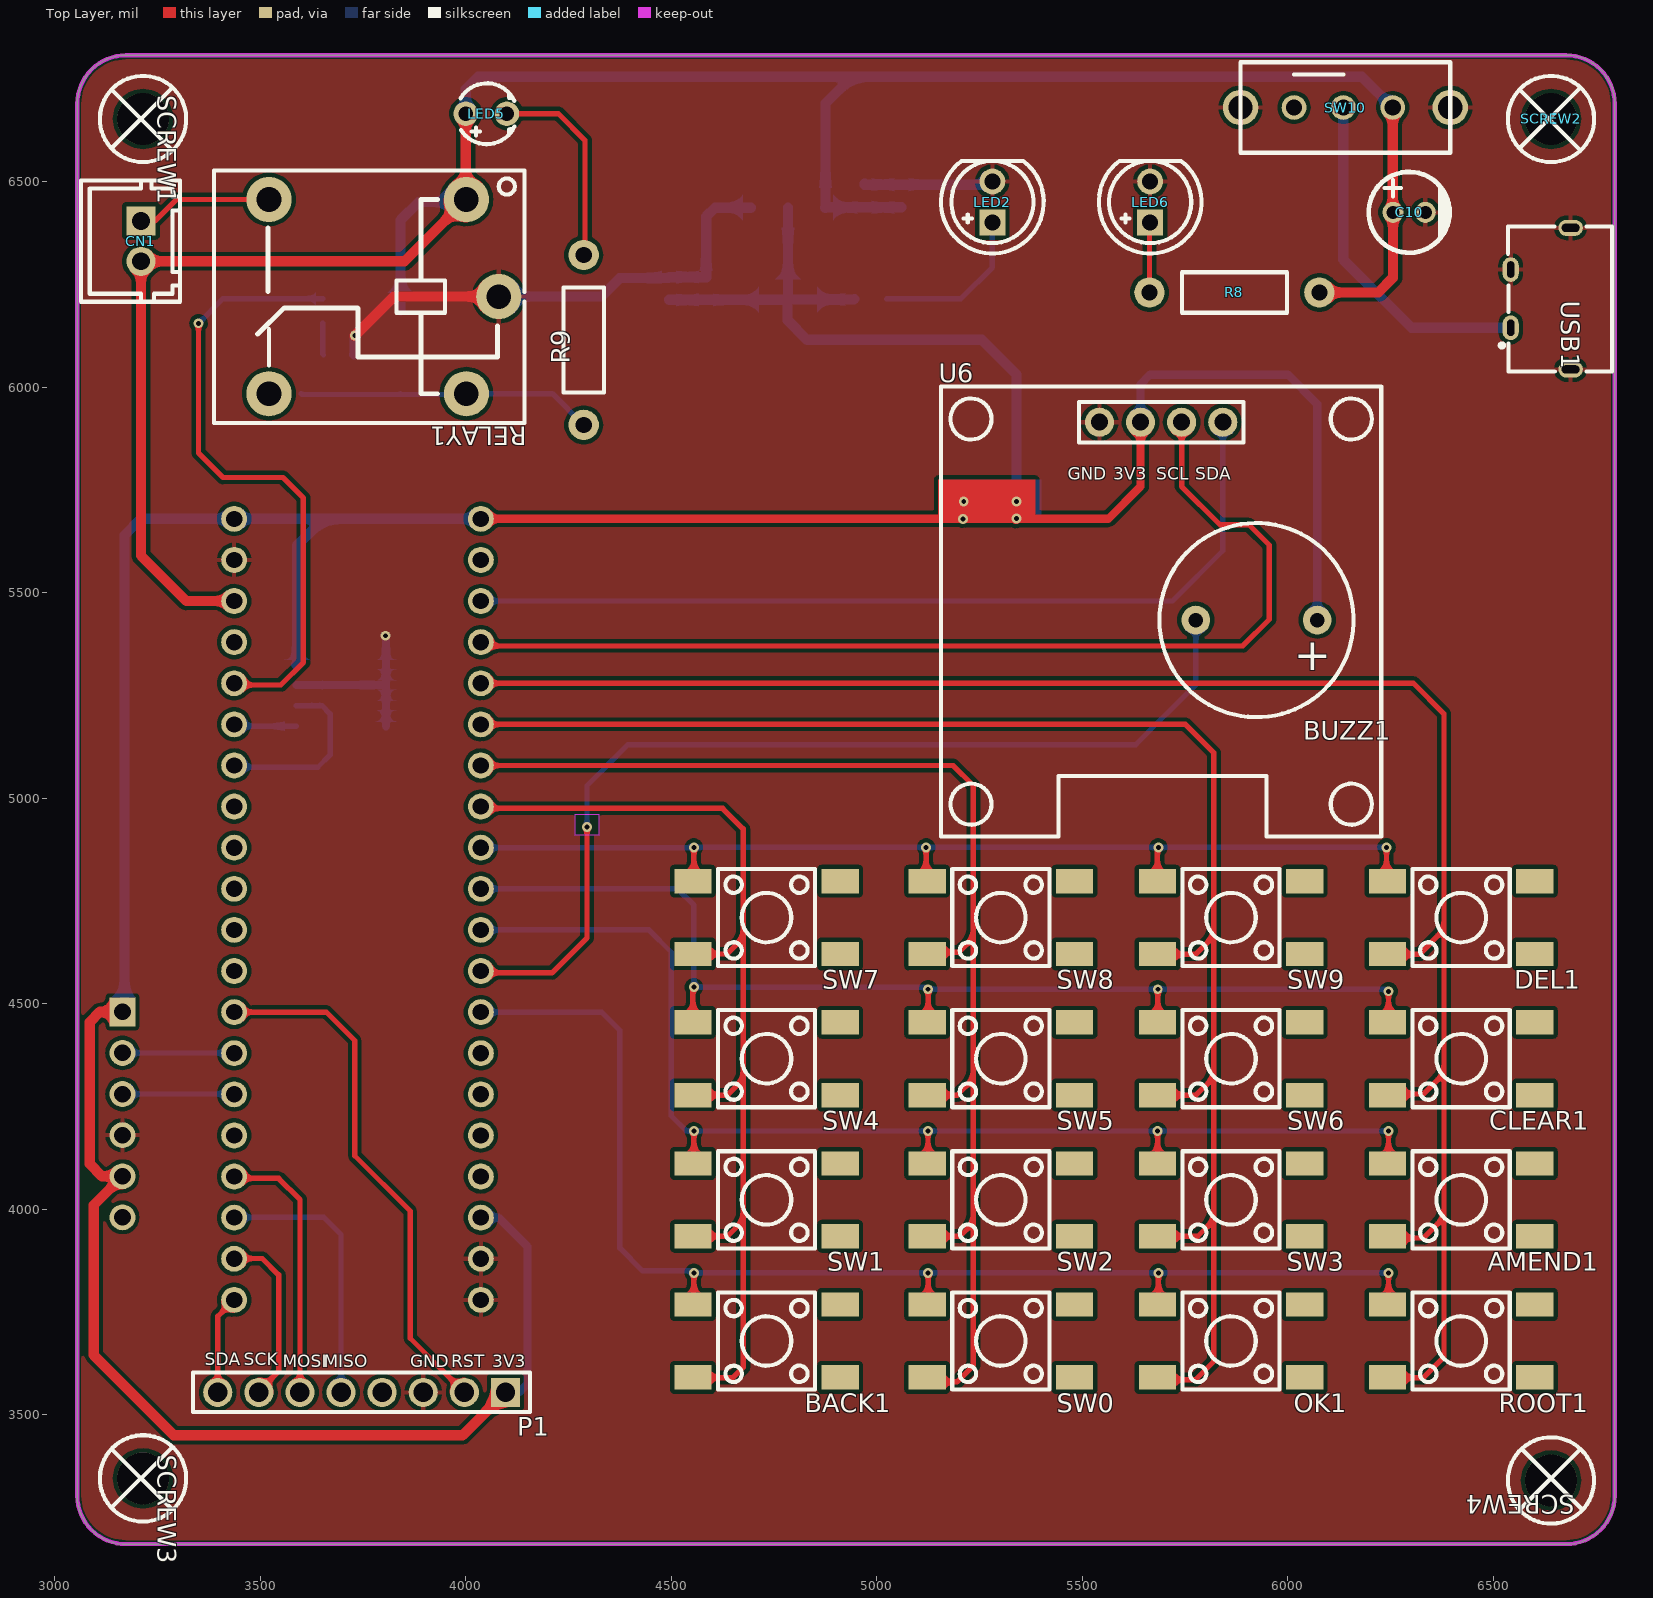
[diagram p0: Top Layer view]
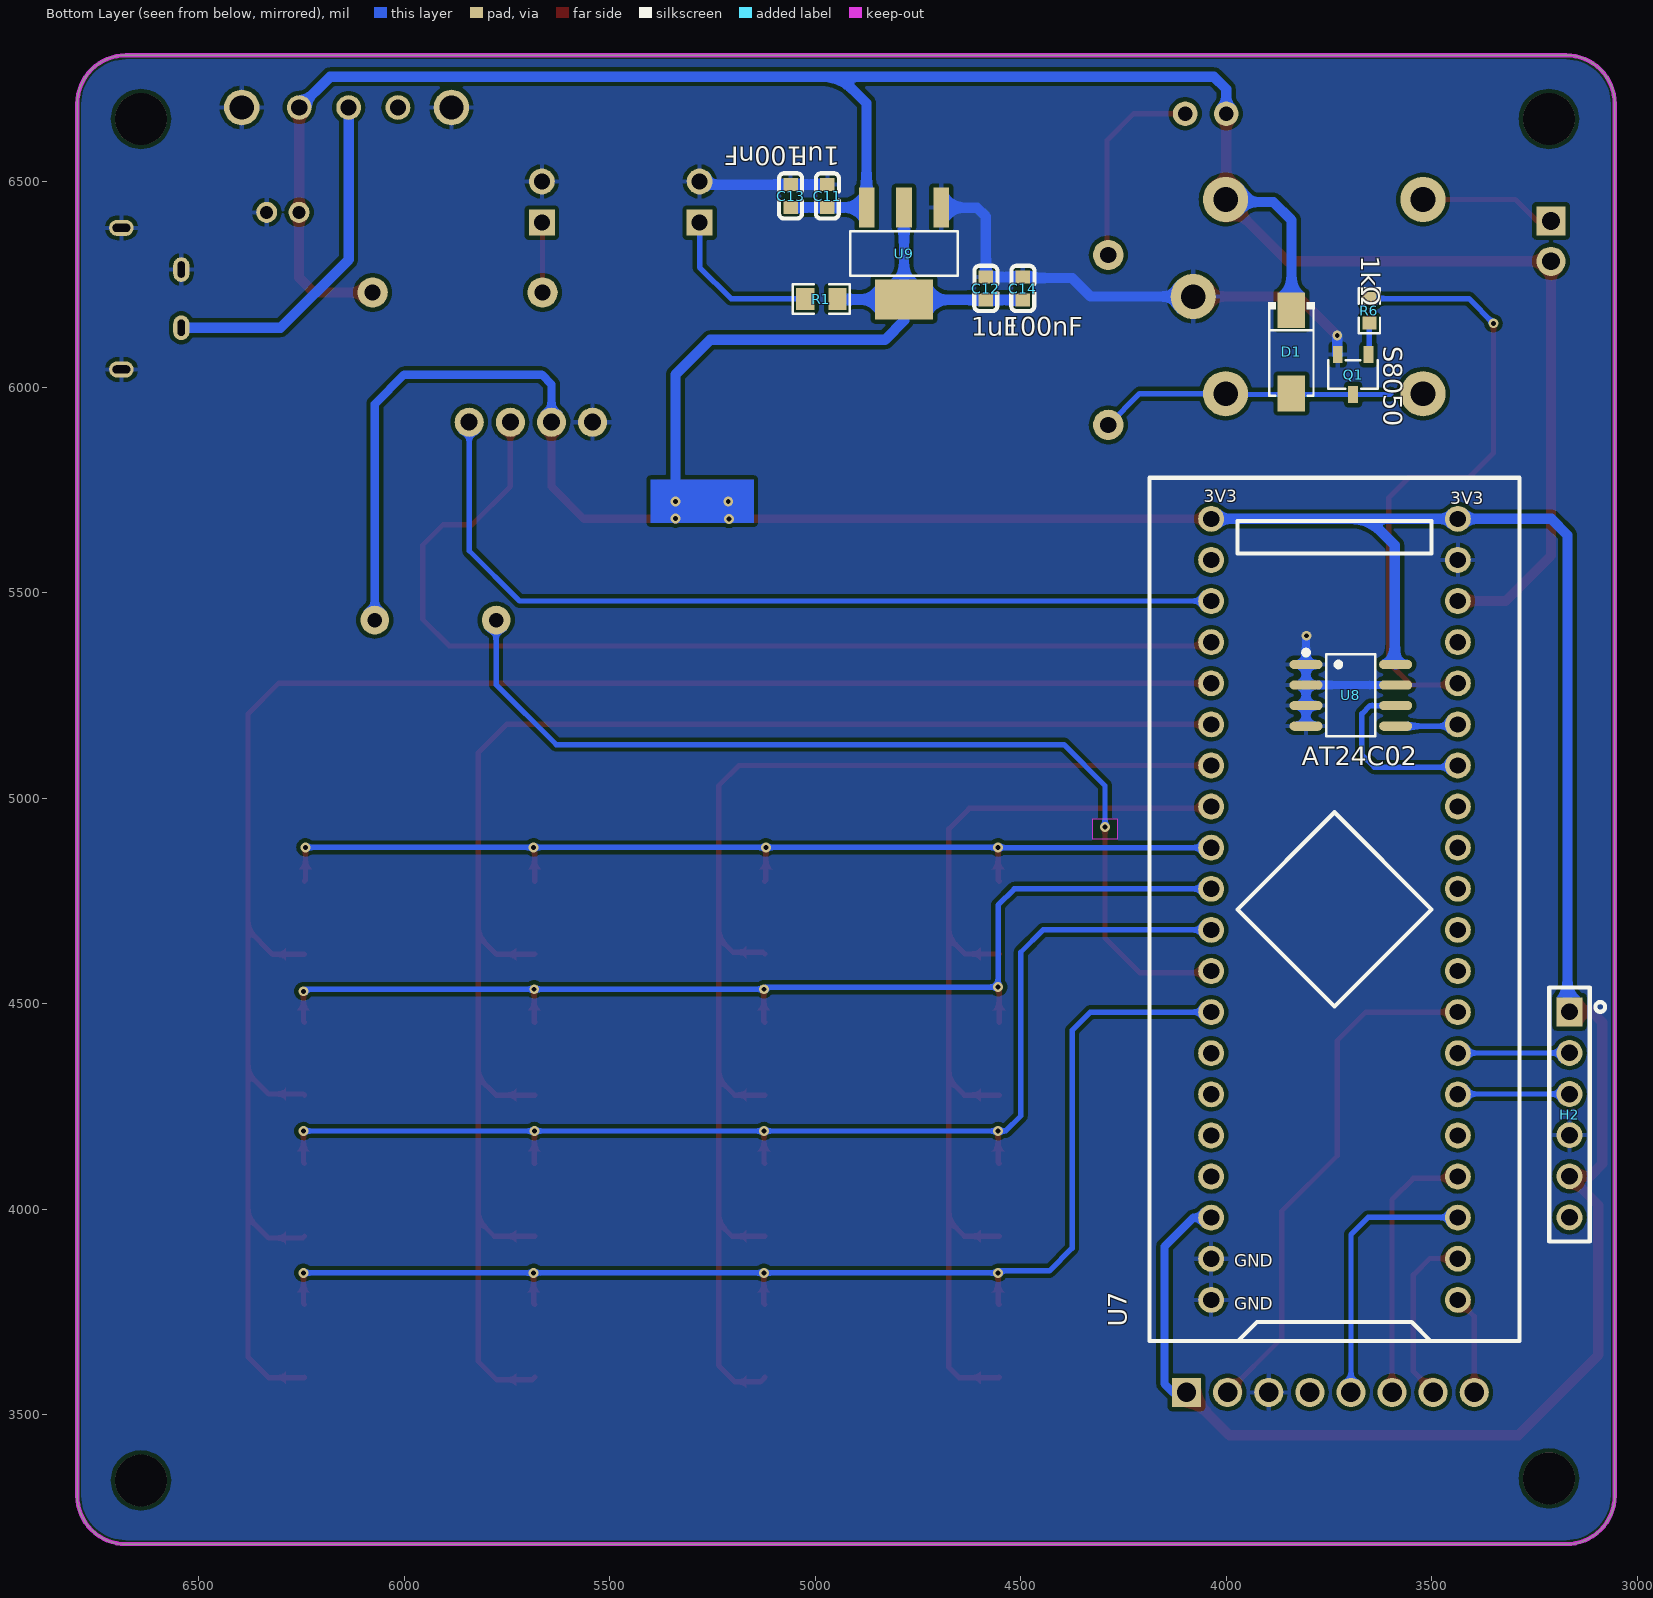
[diagram p1: Bottom Layer view, seen from below]
# Altium PCB MISC61668.pcbdoc
Units mil, origin at the board's own origin, x right, y up, seen from the top; angles counter-clockwise.
Board outline 3740.16 x 3622.05 mil, 2 copper layers (Top Layer, Bottom Layer), stack 62.206 mil thick; 45 components, 31 nets, 185 pads, 24 vias.

## Layer stack, top to bottom
Top Solder Mask Layer: solder mask 0.394, Dk 3.3
Top Layer: signal copper 1.379
Dielectric1: surface 59.449, FR4, Dk 4.5
Bottom Layer: signal copper 1.378
Bottom Solder Mask Layer: solder mask 0.394, Dk 3.3

## Board outline
3173.11,6807.05 ccw(c3173.11,6688.94) 3055,6688.94 3055,3303.11 ccw(c3173.11,3303.11) 3173.11,3185 6677.05,3185 ccw(c6677.05,3303.11) 6795.16,3303.11 6795.16,6688.94 ccw(c6677.05,6688.94) 6677.05,6807.05

## Design rules (kind name [scope] priority, off if disabled: settings)
BoardOutlineClearance copperThickness2oz_1 [All] p2 off: genericclearance=8 ignorepadtopadclearanceinfootprint=FALSE except(0: Arc-SplitContinuation Track-SplitContinuation SMDPad-SplitContinuation THPad-SplitContinuation Via-SplitContinuation Fill-SplitContinuation Region-SplitContinuation Poly-SplitContinuation Text-SplitContinuation Hole-SplitContinuation; 6: Arc-OutlineEdge Track-OutlineEdge SMDPad-OutlineEdge THPad-OutlineEdge Via-OutlineEdge Fill-OutlineEdge Region-OutlineEdge Text-OutlineEdge Hole-OutlineEdge Arc-CutoutEdge Track-CutoutEdge SMDPad-CutoutEdge THPad-CutoutEdge Via-CutoutEdge Fill-CutoutEdge Region-CutoutEdge Text-CutoutEdge Hole-CutoutEdge; 10: Poly-OutlineEdge Poly-CutoutEdge)
BoardOutlineClearance Plane_innerPlane_1 [All] p4 off: genericclearance=8 ignorepadtopadclearanceinfootprint=FALSE except(0: Arc-SplitContinuation Track-SplitContinuation SMDPad-SplitContinuation THPad-SplitContinuation Via-SplitContinuation Fill-SplitContinuation Region-SplitContinuation Poly-SplitContinuation Text-SplitContinuation Hole-SplitContinuation; 6: Arc-OutlineEdge SMDPad-OutlineEdge THPad-OutlineEdge Via-OutlineEdge Fill-OutlineEdge Region-OutlineEdge Text-OutlineEdge Hole-OutlineEdge Arc-CutoutEdge SMDPad-CutoutEdge THPad-CutoutEdge Via-CutoutEdge Fill-CutoutEdge Region-CutoutEdge Text-CutoutEdge Hole-CutoutEdge; 8: Track-OutlineEdge Track-CutoutEdge; 10: Poly-OutlineEdge Poly-CutoutEdge)
BoardOutlineClearance Copper_copperRegion_1 [All] p6 off: genericclearance=8 ignorepadtopadclearanceinfootprint=FALSE except(0: Arc-SplitContinuation Track-SplitContinuation SMDPad-SplitContinuation THPad-SplitContinuation Via-SplitContinuation Fill-SplitContinuation Region-SplitContinuation Poly-SplitContinuation Text-SplitContinuation Hole-SplitContinuation; 6: Arc-OutlineEdge SMDPad-OutlineEdge THPad-OutlineEdge Via-OutlineEdge Fill-OutlineEdge Region-OutlineEdge Text-OutlineEdge Hole-OutlineEdge Arc-CutoutEdge SMDPad-CutoutEdge THPad-CutoutEdge Via-CutoutEdge Fill-CutoutEdge Region-CutoutEdge Text-CutoutEdge Hole-CutoutEdge; 8: Track-OutlineEdge Track-CutoutEdge; 10: Poly-OutlineEdge Poly-CutoutEdge)
BoardOutlineClearance copperThickness1oz_1 [All] p8: genericclearance=8 ignorepadtopadclearanceinfootprint=FALSE except(0: Arc-SplitContinuation Track-SplitContinuation SMDPad-SplitContinuation THPad-SplitContinuation Via-SplitContinuation Fill-SplitContinuation Region-SplitContinuation Poly-SplitContinuation Text-SplitContinuation Hole-SplitContinuation; 6: Arc-OutlineEdge SMDPad-OutlineEdge THPad-OutlineEdge Via-OutlineEdge Fill-OutlineEdge Region-OutlineEdge Text-OutlineEdge Hole-OutlineEdge Arc-CutoutEdge SMDPad-CutoutEdge THPad-CutoutEdge Via-CutoutEdge Fill-CutoutEdge Region-CutoutEdge Text-CutoutEdge Hole-CutoutEdge; 8: Track-OutlineEdge Track-CutoutEdge; 10: Poly-OutlineEdge Poly-CutoutEdge)
Clearance copperThickness2oz [All] p1 off: gap=8 ignorepadtopadclearanceinfootprint=FALSE except(6: SMDPad-Track SMDPad-SMDPad THPad-Track SMDPad-THPad THPad-THPad Track-Via SMDPad-Via THPad-Via Via-Via Fill-Track Region-Track Fill-SMDPad Region-SMDPad Fill-THPad Region-THPad Fill-Via Region-Via Fill-Fill Fill-Region Region-Region Arc-SMDPad Arc-THPad Arc-Via Fill-Arc Region-Arc Arc-Arc Text-Track SMDPad-Text Text-THPad Text-Via Fill-Text Region-Text Text-Text Hole-Track Hole-SMDPad Hole-THPad Hole-Via Fill-Hole Region-Hole Hole-Arc Hole-Text; 10: Poly-Track Poly-SMDPad Poly-THPad Poly-Via Poly-Fill Poly-Region Poly-Poly Poly-Arc Poly-Text Poly-Hole; 11.8: Arc-Track Arc-Text)
Clearance Plane_innerPlane [All] p3 off: gap=8 ignorepadtopadclearanceinfootprint=FALSE except(6: SMDPad-SMDPad SMDPad-THPad THPad-THPad SMDPad-Via THPad-Via Via-Via Fill-SMDPad Region-SMDPad Fill-THPad Region-THPad Fill-Via Region-Via Fill-Fill Fill-Region Region-Region Arc-SMDPad Arc-THPad Arc-Via Fill-Arc Region-Arc Arc-Arc SMDPad-Text Text-THPad Text-Via Fill-Text Region-Text Text-Text Hole-SMDPad Hole-THPad Hole-Via Fill-Hole Region-Hole Hole-Arc Hole-Text; 10: Poly-Track Poly-SMDPad Poly-THPad Poly-Via Poly-Fill Poly-Region Poly-Poly Poly-Arc Poly-Text Poly-Hole; 11.8: Arc-Text)
Clearance Copper_copperRegion [All] p5 off: gap=8 ignorepadtopadclearanceinfootprint=FALSE except(6: SMDPad-SMDPad SMDPad-THPad THPad-THPad SMDPad-Via THPad-Via Via-Via Fill-SMDPad Region-SMDPad Fill-THPad Region-THPad Fill-Via Region-Via Fill-Fill Fill-Region Region-Region Arc-SMDPad Arc-THPad Arc-Via Fill-Arc Region-Arc Arc-Arc SMDPad-Text Text-THPad Text-Via Fill-Text Region-Text Text-Text Hole-SMDPad Hole-THPad Hole-Via Fill-Hole Region-Hole Hole-Arc Hole-Text; 10: Poly-Track Poly-SMDPad Poly-THPad Poly-Via Poly-Fill Poly-Region Poly-Poly Poly-Arc Poly-Text Poly-Hole; 11.8: Arc-Text)
Clearance copperThickness1oz [All] p7: gap=8 ignorepadtopadclearanceinfootprint=FALSE except(6: SMDPad-SMDPad SMDPad-THPad THPad-THPad SMDPad-Via THPad-Via Via-Via Fill-SMDPad Region-SMDPad Fill-THPad Region-THPad Fill-Via Region-Via Fill-Fill Fill-Region Region-Region Arc-SMDPad Arc-THPad Arc-Via Fill-Arc Region-Arc Arc-Arc SMDPad-Text Text-THPad Text-Via Fill-Text Region-Text Text-Text Hole-SMDPad Hole-THPad Hole-Via Fill-Hole Region-Hole Hole-Arc Hole-Text; 10: Poly-Track Poly-SMDPad Poly-THPad Poly-Via Poly-Fill Poly-Region Poly-Poly Poly-Arc Poly-Text Poly-Hole; 11.8: Arc-Text)
DiffPairsRouting differentialPair [All] p1: maxlimit=6 minlimit=6 mostfreqgap=6 toplayer_minwidth=5 toplayer_prefwidth=10 toplayer_maxwidth=100 toplayer_mingap=6 toplayer_prefgap=6 toplayer_maxgap=6 bottomlayer_minwidth=5 bottomlayer_prefwidth=10 bottomlayer_maxwidth=100 bottomlayer_mingap=6 bottomlayer_prefgap=6 bottomlayer_maxgap=6 maxuncoupledlength=10
HoleToHoleClearance otherClearance [All] p1: gap=11.8 allowstackedmicrovias=TRUE
Length netLength [All] p1: minlimit=0 maxlimit=0
PasteMaskExpansion pasteMaskExpansion [All] p1: expansion=0
PlaneConnect innerPlane [All] p1: planeconnectstyle=Relief reliefexpansion=20 reliefentries=4 reliefconductorwidth=10 reliefairgap=10
PolygonConnect copperRegion [All] p1: connectstyle=Relief reliefconductorwidth=10 reliefentries=4 polygonreliefangle="90 Angle" airgapwidth=10 via.connectstyle=Relief via.reliefconductorwidth=10 via.reliefentries=4 via.polygonreliefangle="90 Angle" via.airgapwidth=10
RoutingVias viaSize [All] p1: holewidth=12 width=24 viastyle="Through Hole" minholewidth=11.8 minwidth=19.7 maxholewidth=248 maxwidth=393.7
SolderMaskExpansion solderMaskExpansion [IsVia] p1: expansion=-1000 istentingtop=TRUE
SolderMaskExpansion solderMaskExpansion [All] p2: expansion=2 istentingtop=FALSE
Width copperThickness2oz_2 [(InNet('+3V3') OR InNet('+5V') OR InNet('GND'))] p1: maxlimit=100 minlimit=8 preferedwidth=25
Width copperThickness1oz_2 [All] p2: maxlimit=100 minlimit=5 preferedwidth=13

## Components (designator, comment, footprint, x,y, rotation, side; value= is the part's Value field where it differs from the comment)
AMEND1 "KH-6X6X5H-STM" SW-SMD_4P-L6.0-W6.0-P4.50-LS9.0-2 6421.7,4022.66 r180 top
BACK1 "KH-6X6X5H-STM" SW-SMD_4P-L6.0-W6.0-P4.50-LS9.0-2 4731.7,3679.33 r180 top
BUZZ1 "Buzzer BD12.0-P7.50" BUZ-TH_BD12.0-P7.50-D0.6-FD 5923.78,5433.05 r180 top
C10 "10uF" CAP-TH_BD5.0-P2.00-D0.8-FD 6295,6425 r0 top
C11 "1uF" C0603 4970.55,6464.66 r270 bottom
C12 "1uF" C0603 4585,6239.66 r270 bottom
C13 "100nF" C0603 5060,6464.66 r270 bottom
C14 "100nF" C0603 4495,6239.66 r270 bottom
CLEAR1 "KH-6X6X5H-STM" SW-SMD_4P-L6.0-W6.0-P4.50-LS9.0-2 6421.7,4365.99 r180 top
CN1 "ZX-XH2.54-2PZZ" CONN-TH_2P-P2.50_HX25003-2A 3210,6355 r270 top
D1 "SS14" SMA_L4.2-W2.6-LS5.3-RD 3841.48,6085.3 r270 bottom
DEL1 "KH-6X6X5H-STM" SW-SMD_4P-L6.0-W6.0-P4.50-LS9.0-2 6421.7,4709.33 r180 top
H2 "PM254V-11-06-H85" hdr-th_6p-p2.54-v-f 3165,4230 r270 bottom
LED2 "" LED-TH_5mm 5281.16,6450 r90 top
LED5 "XL-302SURD" LED-TH_BD3.8-P2.54-RD 4050,6665 r180 top
LED6 "" LED-TH_5mm 5665,6450 r90 top
OK1 "KH-6X6X5H-STM" SW-SMD_4P-L6.0-W6.0-P4.50-LS9.0-2 5861.7,3679.33 r180 top
P1 "2.54-1*8P female, RoHS" HDR-TH_8P-P2.54-V-F-1 3746.7,3554.33 r180 top
Q1 "S8050" SOT-23-3_L2.9-W1.6-P1.90-LS2.8-BR 3691.48,6030.3 r90 bottom
R1 "10.1kΩ" R0805 4985,6214.05 r0 bottom
R6 "1kΩ" R0603 3652.01,6185.3 r90 bottom
R8 "1kΩ" RES-TH_BD2.5-L6.5-P10.50-D0.6 5870,6230 r180 top
R9 "1kΩ" RES-TH_BD2.5-L6.5-P10.50-D0.6 4286.91,6114.55 r90 top
RELAY1 "SRD-12VDC-SL-C" RELAY-TH_SRD-XXVDC-XL-C 3800.77,6220.03 r180 top locked
ROOT1 "KH-6X6X5H-STM" SW-SMD_4P-L6.0-W6.0-P4.50-LS9.0-2 6421.7,3679.33 r180 top
SCREW1 "" M3螺丝 3212.48,6649.57 r270 top locked
SCREW2 "" M3螺丝 6637.68,6649.57 r270 top locked
SCREW3 "" M3螺丝 3212.48,3342.48 r270 top locked
SCREW4 "" M3螺丝 6637.68,3342.48 r180 top locked
SW0 "KH-6X6X5H-STM" SW-SMD_4P-L6.0-W6.0-P4.50-LS9.0-2 5301.7,3679.33 r180 top
SW1 "KH-6X6X5H-STM" SW-SMD_4P-L6.0-W6.0-P4.50-LS9.0-2 4731.7,4022.66 r180 top
SW2 "KH-6X6X5H-STM" SW-SMD_4P-L6.0-W6.0-P4.50-LS9.0-2 5301.7,4022.66 r180 top
SW3 "KH-6X6X5H-STM" SW-SMD_4P-L6.0-W6.0-P4.50-LS9.0-2 5861.7,4022.66 r180 top
SW4 "KH-6X6X5H-STM" SW-SMD_4P-L6.0-W6.0-P4.50-LS9.0-2 4731.7,4365.99 r180 top
SW5 "KH-6X6X5H-STM" SW-SMD_4P-L6.0-W6.0-P4.50-LS9.0-2 5301.7,4365.99 r180 top
SW6 "KH-6X6X5H-STM" SW-SMD_4P-L6.0-W6.0-P4.50-LS9.0-2 5861.7,4365.99 r180 top
SW7 "KH-6X6X5H-STM" SW-SMD_4P-L6.0-W6.0-P4.50-LS9.0-2 4731.7,4709.33 r180 top locked
SW8 "KH-6X6X5H-STM" SW-SMD_4P-L6.0-W6.0-P4.50-LS9.0-2 5301.7,4709.33 r180 top
SW9 "KH-6X6X5H-STM" SW-SMD_4P-L6.0-W6.0-P4.50-LS9.0-2 5861.7,4709.33 r180 top
SW10 "SK-12E12-G5" SW-TH_SK-12E12-G5 6140,6680 r90 top
U6 "HS96L03W2C03" OLED-TH_L27.8-W27.2-P2.54_C9900033791 5691.7,5914.33 r0 top
U7 "STM32F103C8T6-Card" CONN-TH_L53.3-W22.9_STM32F103C8T6-CARD 3736.7,4729.33 r90 bottom locked
U8 "AT24C02" SOP-8_L5.0-W4.0-P1.27-LS6.0-BL 3696.96,5250 r270 bottom
U9 "AMS1117-3.3" SOT-223-4_L6.5-W3.5-P2.30-LS7.0-BR 4783.95,6324.77 r90 bottom
USB1 "KH-TYPE-C-2P" USB-SMD_KH-TYPE-C-2P 6615,6215 r90 top

## Footprints (in the part's own frame and the unit in brackets; to place one, negate y for a bottom-side part, rotate by r counter-clockwise, add the part's x,y. Pads: shape width x height; smd on the part's side, far side on the other; paste and mask are expansions set on the pad)
BUZ-TH_BD12.0-P7.50-D0.6-FD [mil]
  round 70 hole 35.43: 1(-147.64,0) 2(147.64,0)
  silkscreen extent -236,-236 236,236
C0603 [mm]
  rect 0.8x0.9 smd: 1(-0.7,0) 2(0.7,0)
  silkscreen extent -1.41,-0.71 1.39,0.72
CAP-TH_BD5.0-P2.00-D0.8-FD [mm]
  round 1.3 hole 0.8: 1(-1,0) 2(1,0)
  silkscreen extent -2.5,-2.5 2.5,2.5
CONN-TH_2P-P2.50_HX25003-2A [mm]
  rect 1.8x1.8 hole 1.1 paste+0 mask+0.05: 1(-1.25,0)
  round 1.8 hole 1.1 paste+0 mask+0.05: 2(1.25,0)
  silkscreen extent -3.75,-3.7 3.75,2.41
CONN-TH_L53.3-W22.9_STM32F103C8T6-CARD [mm]
  round 1.6 hole 1: 1(-24.13,-7.62) 2(-21.59,-7.62) 3(-19.05,-7.62) 4(-16.51,-7.62) 5(-13.97,-7.62) 6(-11.43,-7.62) 7(-8.89,-7.62) 8(-6.35,-7.62) 9(-3.81,-7.62) 10(-1.27,-7.62) 11(1.27,-7.62) 12(3.81,-7.62) 13(6.35,-7.62) 14(8.89,-7.62) 15(11.43,-7.62) 16(13.97,-7.62) 17(16.51,-7.62) 18(19.05,-7.62) 19(21.59,-7.62) 20(24.13,-7.62) 21(24.13,7.62) 22(21.59,7.62) 23(19.05,7.62) 24(16.51,7.62) 25(13.97,7.62) 26(11.43,7.62) 27(8.89,7.62) 28(6.35,7.62) 29(3.81,7.62) 30(1.27,7.62) 31(-1.27,7.62) 32(-3.81,7.62) 33(-6.35,7.62) 34(-8.89,7.62) 35(-11.43,7.62) 36(-13.97,7.62) 37(-16.51,7.62) 38(-19.05,7.62) 39(-21.59,7.62) 40(-24.13,7.62)
  silkscreen extent -26.67,-11.43 26.67,11.43
hdr-th_6p-p2.54-v-f [mm]
  rect 1.8x1.6 hole 1.02: 1(-6.35,0)
  round 1.6 hole 1.02: 2(-3.81,0) 3(-1.27,0) 4(1.27,0) 5(3.81,0) 6(6.35,0)
  silkscreen extent -7.85,-1.25 7.85,2.2
HDR-TH_8P-P2.54-V-F-1 [mm]
  rect 1.8x1.8 hole 1.2: 1(-8.89,0)
  round 1.8 hole 1.2: 2(-6.35,0) 3(-3.81,0) 4(-1.27,0) 5(1.27,0) 6(3.81,0) 7(6.35,0) 8(8.89,0)
  silkscreen extent -10.41,-1.22 10.41,1.22
LED-TH_5mm [mm]
  rect 1.6x1.6 hole 1 paste+0 mask+0.051: 1(-1.27,0)
  round 1.6 hole 1 paste+0 mask+0.051: 2(1.27,0)
  silkscreen extent -3.17,-3.17 2.54,3.17
LED-TH_BD3.8-P2.54-RD [mil]
  round 60 hole 35.43: 1(-50,0) 2(50,0)
  silkscreen extent -68,-74 63,74
M3螺丝 [mil]
  round 126 hole 126 paste+0 mask+4: 1(-2.5,2.5)
  silkscreen extent -107,-102 102,107
OLED-TH_L27.8-W27.2-P2.54_C9900033791 [mm]
  round 1.8 hole 1.05 paste+0 mask+0.05: 1(-3.81,0) 2(-1.27,0) 3(1.27,0) 4(3.81,0)
  silkscreen extent -13.6,-25.6 13.6,2.2
R0603 [mil]
  rect 31.75x34.02 smd paste-3937.01 mask+2: 1(-29.66,0) 2(29.66,0)
  silkscreen extent -55,-26 55,26
R0805 [mm]
  rect 1.133x1.377 smd paste-100 mask+0.051: 1(-1,0) 2(1,0)
  silkscreen extent -1.76,-0.92 1.76,0.92
RELAY-TH_SRD-XXVDC-XL-C [mil]
  round 110 hole 60: 1(-200.79,-236.22) 2(279.53,-236.2) 3(279.53,236.2) 4(-200.79,236.22) 5(-279.53,0)
  silkscreen extent -342,-307 413,307
RES-TH_BD2.5-L6.5-P10.50-D0.6 [mil]
  round 74 hole 39.37: 1(-206.69,0) 2(206.69,0)
  silkscreen extent -128,-49 128,49
SMA_L4.2-W2.6-LS5.3-RD [mm]
  rect 2.2x1.7 smd: 1(-2.565,0) 2(2.565,0)
  silkscreen extent -3.08,-1.44 2.7,1.44
SOP-8_L5.0-W4.0-P1.27-LS6.0-BL [mil]
  oval 22.6x80.14 smd: 1(-75,-108.97) 2(-25,-108.97) 3(25,-108.97) 4(75,-108.97) 5(75,108.97) 6(25,108.97) 7(-25,108.97) 8(-75,108.97)
  silkscreen extent -110,-115 99,60
SOT-23-3_L2.9-W1.6-P1.90-LS2.8-BR [mm]
  rect 1.07x0.6 smd: 1(1.235,-0.95) 2(1.235,0.95) 3(-1.235,0)
  silkscreen extent -0.88,-1.54 0.88,1.54
SOT-223-4_L6.5-W3.5-P2.30-LS7.0-BR [mm]
  rect 2.47x0.98 smd: 1(2.835,-2.3) 2(2.835,0) 3(2.835,2.3)
  rect 2.47x3.6 smd: 4(-2.835,0)
  silkscreen extent -1.37,-3.33 1.37,3.33
SW-SMD_4P-L6.0-W6.0-P4.50-LS9.0-2 [mm]
  rect 2.3x1.5 smd: 1(-4.55,2.25) 2(4.55,2.25) 3(-4.55,-2.25) 4(4.55,-2.25)
  silkscreen extent -3,-3 3,3
SW-TH_SK-12E12-G5 [mil]
  round 60 hole 39.37: 1(0,125) 2(0,5) 3(0,-115)
  round 86.61 hole 59.06: 4(0,-255) 5(0,255)
  silkscreen extent -110,-255 110,255
USB-SMD_KH-TYPE-C-2P [mm]
  oval 1.524x1 hole 0.45 slot 1 at 0 deg paste+0 mask+0.05: 1(-1.8,1.85) 2(1.8,1.85)
  oval 1x1.524 hole 0.5 slot 1.1 at 90 deg paste+0 mask+0.05: 3(4.375,-1.85) 4(-4.375,-1.85)
  silkscreen extent -4.5,-4.41 4.46,2.53

## Via types
v1: diameter 24, hole 12, Top Layer to Bottom Layer, 24 vias

## Nets (pads, with @x,y where several pads share a name; then routed paths per layer and width w, separated by ;. In a path a pad name is that pad's centre, name@x,y a point inside that pad or via, vN(x,y) a via of type N, cw(c..) or ccw(c..) an arc to the next point about the centre after c; other vN are vias at no path point)
$1N2265: LED2.1 R1.2 | length 397.6
  Bottom Layer w13: R1.2 5025.32,6215 5205,6215 5281.16,6291.16 LED2.1
$1N4836: CN1.1 RELAY1.2 | length 332.8
  Top Layer w13: CN1.1 3244.21,6404.21 3296.23,6456.23 RELAY1.2
$1N5221: D1.2 Q1.3 R9.1 RELAY1.4 | length 723.9
  Bottom Layer w13: 3599.98,5983.81 3602.1,5981.68 Q1.3 D1.2@3838.86,5981.68 ; D1.2 D1.2@3838.86,5981.68 ; R9.1 4210.96,5983.81 RELAY1.4 3999.43,5981.68 D1.2@3838.86,5981.68
$1N5245: Q1.1 R6.1 | length 77.6
  Bottom Layer w13: R6.1 3652.01,6081 Q1.1
$1N11459: SW10.2 USB1.1 | length 845.9
  Bottom Layer w25: SW10.2 6135,6310 6300.87,6144.13 USB1.1
$1N11461: LED6.1 R8.2 | length 170.7
  Top Layer w13: R8.2 5663.31,6398.31 LED6.1
$1N12136: LED5.1 R9.2 | length 497
  Top Layer w13: LED5.1 4225,6665 4290,6600 4290,6324.33 R9.2
+3V3: BUZZ1.1 C12.2 C14.2 H2.1 H2.5 P1.1 R1.1 U6.2 U7.20 U7.21 U7.38 U8.8 U9.2 U9.4 | length 9651
  Top Layer w20: U7.21 v1(5209.89,5679.33) v1@5337.73,5679.33 ; v1@5339.33,5679.33 5563.05,5679.33 5641.7,5757.97 U6.2
  Top Layer w25: H2.1 3110,4480 3085,4455 3085,4110 3115,4080 H2.5 3095,4010 3095,3645 3290,3450 3992.37,3450 P1.1 ; v1@5337.73,5679.33 5339.33,5679.33 v1(5340,5680)
  Bottom Layer w20: U7.38 4080,3979.33 4150,3909.33 4150,3575 4129.33,3554.33 P1.1 ; U6.2 5641.7,6006.7 5665,6030 6000,6030 6071.42,5958.58 BUZZ1.1
  Bottom Layer w25: H2.1 3170,4485 3170,5640 3209.33,5679.33 U7.20 3654.2,5679.33 ; U8.8 3590,5327.01 3590,5615.13 3654.2,5679.33 ; U7.21 3654.2,5679.33 ; C14.2 C12.2 U9.4@4782.9,6212.1 ; U9.2 U9.4 ; R1.1 4944.74,6213.16 U9.4 ; v1(5340,5680) v1(5340,5721.21) 5340,6030 5255,6115 4830,6115 4782.9,6162.1 U9.4@4782.9,6212.1 ; U9.4@4782.9,6212.1 U9.4
  other v1: 5211.47,5721.21
+5V: C10.1 C11.2 C13.2 CN1.2 D1.1 LED5.2 R8.1 RELAY1.1 SW10.3 U7.18 U9.3 | length 5949.8
  Top Layer w25: U7.18 3320.67,5479.33 3210,5590 CN1.2 3851.1,6305.79 RELAY1.1 4000,6457.8 LED5.2 ; R8.1 6220,6230 6255.63,6265.63 C10.1 6255,6425.63 SW10.3
  Bottom Layer w25: D1.1 3841.48,6406.48 3885,6450 3995.31,6450 RELAY1.1 ; LED5.2 4000,6725 4030,6755 4940,6755 ; U9.3 U9.3@4875.23,6437.1 ; C13.2 C11.2 U9.3@4875.23,6437.1 ; SW10.3 6180,6755 4940,6755 ; U9.3@4875.23,6437.1 4875.23,6690.23 4940,6755
BUZZER_PA7: BUZZ1.2 U7.32 | length 2405.3
  Top Layer w13: U7.32 4041.03,4575 4210,4575 4295,4660 v1(4295,4930)
  Bottom Layer w13: v1(4295,4930) 4295,5030 4395,5130 5630,5130 5776.14,5276.14 BUZZ1.2
GND: C10.2 C11.1 C12.1 C13.1 C14.1 H2.4 LED2.2 LED6.2 P1.3 Q1.2 RELAY1.5 SW10.4 SW10.5 U6.1 U7.19 U7.39 U7.40 U8.1 U8.2 U8.3 U8.4 U8.7 U9.1 USB1.2 USB1.3 USB1.4 | length 1980.8
  Top Layer w25: v1(3730,6125) 3825.03,6220.03 RELAY1.5
  Bottom Layer w20: U8.7 U8.2 ; v1(3805,5395) 3805.93,5394.07 U8.1 U8.2 ; U8.4 U8.3 U8.2
  Bottom Layer w25: Q1.2 3730,6080.04 v1(3730,6125) ; RELAY1.5 4330.03,6220.03 4375,6265 4492.77,6265 C14.1 C12.1 4585,6415 4606.38,6436.38 U9.1 ; C11.1 4970.55,6494.45 4972.77,6492.23 C13.1 5273.39,6492.23 LED2.2
K1_PB8: R6.2 U7.16 | length 1535.3
  Top Layer w13: v1(3350,6155) 3350,5840 3410,5780 3555,5780 3605,5730 3605,5330 3550,5275 3441.03,5275 U7.16
  Bottom Layer w13: v1(3350,6155) 3409.96,6214.96 R6.2
KEY1: AMEND1.2 CLEAR1.2 DEL1.2 ROOT1.2 U7.25 | length 4579.2
  Top Layer w13: U7.25 6305.67,5279.33 6380,5205 6380,4680 ; ROOT1.2 6243.32,3590 6330,3590 6380,3640 6380,3980 ; AMEND1.2 6246.65,3930 6330,3930 6380,3980 ; CLEAR1.2 6245.15,4280 6330,4280 6380,4330 ; DEL1.2 6243.32,4620 6320,4620 6380,4680 ; 6380,3980 6380,4330 ; 6380,4330 6380,4680
KEY2: OK1.2 SW3.2 SW6.2 SW9.2 U7.26 | length 3915.9
  Top Layer w13: U7.26 5750.67,5179.33 5820,5110 5820,4665 ; OK1.2 5688.32,3585 5775,3585 5820,3630 5820,3973.21 ; SW3.2 5780.87,3934.09 5820,3973.21 ; SW6.2 5776.69,4277.42 5820,4320.73 ; SW9.2 5683.32,4620 5775,4620 5820,4665 ; 5820,3973.21 5820,4320.73 ; 5820,4320.73 5820,4665
KEY3: SW0.2 SW2.2 SW5.2 SW8.2 U7.27 | length 3145.6
  Top Layer w13: U7.27 5185.67,5079.33 5235,5030 5235,4660 ; SW0.2 5133.32,3580 5195,3580 5235,3620 5235,3966.99 ; SW2.2 5202.09,3934.09 5235,3966.99 ; SW5.2 5195.77,4277.42 5235,4316.65 ; SW8.2 5126.81,4625 5200,4625 5235,4660 ; 5235,3966.99 5235,4316.65 ; 5235,4316.65 5235,4660
KEY4: BACK1.2 SW1.2 SW4.2 SW7.2 U7.28 | length 2518.9
  Top Layer w13: U7.28 4041.03,4975 4625,4975 4675,4925 4675,4660 ; BACK1.2 4553.32,3590 4650,3590 4675,3615 4675,3972.03 ; SW1.2 4637.06,3934.09 4675,3972.03 ; SW4.2 4637.14,4277.42 4675,4315.28 ; SW7.2 4635.75,4620.75 4675,4660 ; 4675,3972.03 4675,4315.28 ; 4675,4315.28 4675,4660
KEY5: DEL1.4 SW7.4 SW8.4 SW9.4 U7.29 | length 2536.1
  Top Layer w13: SW7.4 4555,4800.35 v1(4555,4880) ; v1(5120,4880) 5120,4800.48 SW8.4 ; SW9.4 5682.57,4877.57 v1(5685,4880) ; v1(6240,4880) 6240,4800.48 DEL1.4
  Bottom Layer w13: U7.29 4554.33,4879.33 v1(4555,4880) v1(5120,4880) v1(5685,4880) v1(6240,4880)
KEY6: CLEAR1.4 SW4.4 SW5.4 SW6.4 U7.30 | length 2753.9
  Top Layer w13: SW4.4 4552.57,4537.57 v1(4555,4540) ; SW5.4 5125,4457.01 v1(5125,4535) ; SW6.4 5683.64,4455.65 v1(5683.64,4535) ; CLEAR1.4 6245,4457.01 v1(6245,4530)
  Bottom Layer w13: U7.30 4515.67,4779.33 4555,4740 v1(4555,4540) 5120,4540 v1(5125,4535) v1(5683.64,4535) 6240,4535 v1(6245,4530)
KEY7: AMEND1.4 SW1.4 SW2.4 SW3.4 U7.31 | length 2962.5
  Top Layer w13: SW1.4 4555,4113.68 v1(4555,4190) ; SW2.4 5124.53,4113.21 v1(5124.53,4190) ; SW3.4 5683.16,4111.84 v1(5683.16,4190) ; AMEND1.4 6245,4113.68 v1(6245,4190)
  Bottom Layer w13: U7.31 4445.67,4679.33 4500,4625 4500,4226.62 4536.62,4190 v1(4555,4190) v1(5124.53,4190) v1(5683.16,4190) v1(6245,4190)
KEY8: BACK1.4 OK1.4 ROOT1.4 SW0.4 U7.33 | length 3093.9
  Top Layer w13: BACK1.4 4555,3770.35 v1(4555,3845) ; SW0.4 5125,3770.35 v1(5125,3845) ; OK1.4 5685,3770.35 v1(5685,3845) ; ROOT1.4 6245,3770.35 v1(6245,3845)
  Bottom Layer w13: U7.33 4330.67,4479.33 4375,4435 4375,3905 4430,3850 4550,3850 v1(4555,3845) v1(5125,3845) v1(5685,3845) v1(6245,3845)
OLED_SCL: U6.3 U7.24 | length 2557.8
  Top Layer w13: U7.24 4046.03,5370 5890,5370 5955,5435 5955,5615 5905,5665 5835,5665 5741.7,5758.3 U6.3
OLED_SDA: U6.4 U7.23 | length 2168.3
  Bottom Layer w13: U7.23 5719.33,5479.33 5841.7,5601.7 U6.4
PB6_SCL: U7.14 U8.6 | length 437.8
  Bottom Layer w13: U7.14 3441.03,5075 3640,5075 3670,5105 3670,5205 3650,5225 U8.6
PB7_SDA: U7.15 U8.5 | length 153.1
  Bottom Layer w13: U7.15 3441.03,5175 U8.5
PB12_SDA: P1.8 U7.1 | length 241.6
  Top Layer w13: P1.8 3396.7,3739.33 U7.1
PB13_SCK: P1.7 U7.2 | length 430.8
  Top Layer w13: U7.2 3437.37,3880 3505,3880 3545,3840 3545,3605 3496.7,3556.7 P1.7
PB14_MISO: P1.5 U7.3 | length 661.5
  Bottom Layer w13: U7.3 3437.37,3980 3655,3980 3696.7,3938.3 P1.5
PB15_MOSI: P1.6 U7.4 | length 652.2
  Top Layer w13: U7.4 3441.03,4075 3545,4075 3596.7,4023.3 P1.6
RST: P1.2 U7.8 | length 1288.2
  Top Layer w13: U7.8 3660.67,4479.33 3730,4410 3730,4130 3865,3995 3865,3686.02 P1.2
RX_PA9_TX1: H2.3 U7.6 | length 272
  Bottom Layer w13: H2.3 3436.03,4280 U7.6
TX_PA10_RX1: H2.2 U7.7 | length 272
  Bottom Layer w13: H2.2 3436.03,4380 U7.7
pads on no net: AMEND1.1 AMEND1.3 BACK1.1 BACK1.3 CLEAR1.1 CLEAR1.3 DEL1.1 DEL1.3 H2.6 OK1.1 OK1.3 P1.4 RELAY1.3 ROOT1.1 ROOT1.3 SCREW1.1 SCREW2.1 SCREW3.1 SCREW4.1 SW0.1 SW0.3 SW1.1 SW1.3 SW2.1 SW2.3 SW3.1 SW3.3 SW4.1 SW4.3 SW5.1 SW5.3 SW6.1 SW6.3 SW7.1 SW7.3 SW8.1 SW8.3 SW9.1 SW9.3 SW10.1 U7.5 U7.9 U7.10 U7.11 U7.12 U7.13 U7.17 U7.22 U7.34 U7.35 U7.36 U7.37

## Polygon pours and split planes (outlines as drawn)
GND on Top Layer (solid, remove dead copper, pour order 0): 3000,6845 3000,3155 6840,3155 6840,6845
GND on Bottom Layer (solid, remove dead copper, pour order 2): 3050,6925 3050,3000 6815,3000 6815,6925

## Keep-outs
Top Layer:
  region: 4265,4960 4265,4910.4 4325,4910.4 4325,4960
Bottom Layer:
  region: 4265,4950 4265,4900 4325,4900 4325,4950
Board Outline Layer:
  the board outline again, w10

## Other copper
Top Layer:
  drawing of 98 lines, arcs and shapes, not listed
Bottom Layer:
  drawing of 101 lines, arcs and shapes, not listed

## Silkscreen, mask and mechanical layers (free items; w line width, h text height)
Top Silkscreen Layer:
  text "GND" at 5465,5775 h30
  text "3V3" at 5575,5775 h30
  text "SCL" at 5680,5775 h30
  text "SDA" at 5775,5775 h30
  text "SDA" at 3365,3620 h30
  text "SCK" at 3460,3620 h30
  text "MOSI" at 3555,3615 h30
  text "MISO" at 3655,3615 h30
  text "GND" at 3865,3615 h30
  text "RST" at 3965,3615 h30
  text "3V3" at 4065,3615 h30
Bottom Silkscreen Layer:
  text "3V3" at 4055,5720 h30
  text "3V3" at 3455,5715 h30
  text "GND" at 3980,3860 h30
  text "GND" at 3980,3755 h30